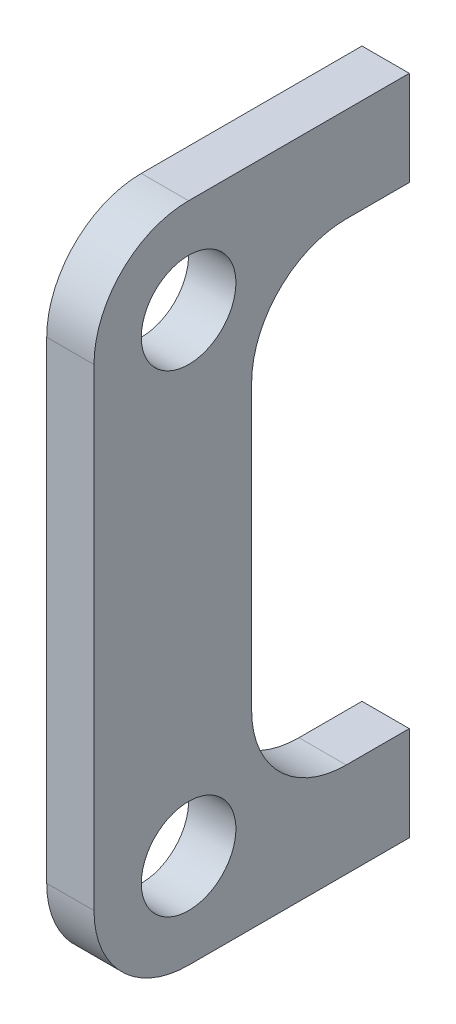
SolidWorks part; units mm, degrees
ref_plane "Front Plane" through (0, 0, 0) normal (0, 0, 1) x (1, 0, 0)
ref_plane "Top Plane" through (0, 0, 0) normal (0, 1, 0) x (1, 0, 0)
ref_plane "Right Plane" through (0, 0, 0) normal (1, 0, 0) x (0, 0, -1)
other "Configuration Table"
sketch "Sketch2" plane through (-215.4122, 0, 0) normal (-1, 0, 0) x (0, 0, 1)
  line L0 (0, -13) -> (20, -13)
  line L1 (50, 17) -> (50, 107)
  line L2 (20, 137) -> (0, 137)
  line L3 (0, 137) -> (0, 167)
  line L4 (0, 167) -> (70, 167)
  line L5 (100, 137) -> (100, -13)
  line L6 (0, -13) -> (0, -43)
  line L7 (70, -43) -> (0, -43)
  arc A0 (70, 167) -> (100, 137) centre (70, 137) cw
  arc A1 (100, -13) -> (70, -43) centre (70, -13) cw
  arc A2 (50, 107) -> (20, 137) centre (20, 107) ccw
  arc A3 (20, -13) -> (50, 17) centre (20, 17) ccw
  point P17 (100, -43)
  point P20 (50, 137)
  point P23 (50, -13)
  dimension "D4" = 30
  dimension "D5" = 30
  dimension "D1" = 100
  dimension "D2" = 150
  dimension "D3" = 50
extrude "Boss-Extrude1" add sketch "Sketch2" along normal up to surface (175.6234 mm away)
sketch "Sketch3" plane through (-230.4122, 0, 0) normal (-1, 0, 0) x (0, 0, 1)
  circle A0 centre (70, -13) radius 15
  circle A1 centre (70, 137) radius 15
  dimension "D1" = 30
extrude "Cut-Extrude1" cut sketch "Sketch3" against normal through all both and the other way through all
